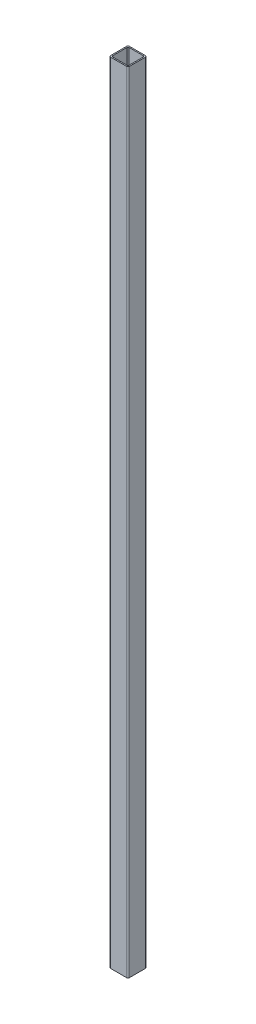
SolidWorks part; units mm, degrees
material "Angle steel 100×100×6/Q235"
ref_plane "Front Plane" through (0, 0, 0) normal (0, 0, 1) x (1, 0, 0)
ref_plane "Top Plane" through (0, 0, 0) normal (0, 1, 0) x (1, 0, 0)
ref_plane "Right Plane" through (0, 0, 0) normal (1, 0, 0) x (0, 0, -1)
sketch "Sketch2" plane through (0, 0, 0) normal (0, 1, 0) x (1, 0, 0)
  line L0 (12.6, 4.775) -> (87.4, 4.775)
  line L1 (6.3, 11.075) -> (6.3, 85.875)
  line L2 (87.4, 92.175) -> (12.6, 92.175)
  line L3 (93.7, 85.875) -> (93.7, 11.075)
  line L4 (7.875, -1.525) -> (92.125, -1.525)
  line L5 (0, 6.35) -> (0, 90.6)
  line L6 (92.125, 98.475) -> (7.875, 98.475)
  line L7 (100, 90.6) -> (100, 6.35)
  arc A0 (100, 90.6) -> (92.125, 98.475) centre (92.125, 90.6) ccw
  arc A1 (92.125, -1.525) -> (100, 6.35) centre (92.125, 6.35) ccw
  arc A2 (0, 6.35) -> (7.875, -1.525) centre (7.875, 6.35) ccw
  arc A3 (7.875, 98.475) -> (0, 90.6) centre (7.875, 90.6) ccw
  arc A4 (12.6, 92.175) -> (6.3, 85.875) centre (12.6, 85.875) ccw
  arc A5 (93.7, 85.875) -> (87.4, 92.175) centre (87.4, 85.875) ccw
  arc A6 (87.4, 4.775) -> (93.7, 11.075) centre (87.4, 11.075) ccw
  arc A7 (6.3, 11.075) -> (12.6, 4.775) centre (12.6, 11.075) ccw
extrude "Boss-Extrude1" add sketch "Sketch2" along normal mid plane 4200
